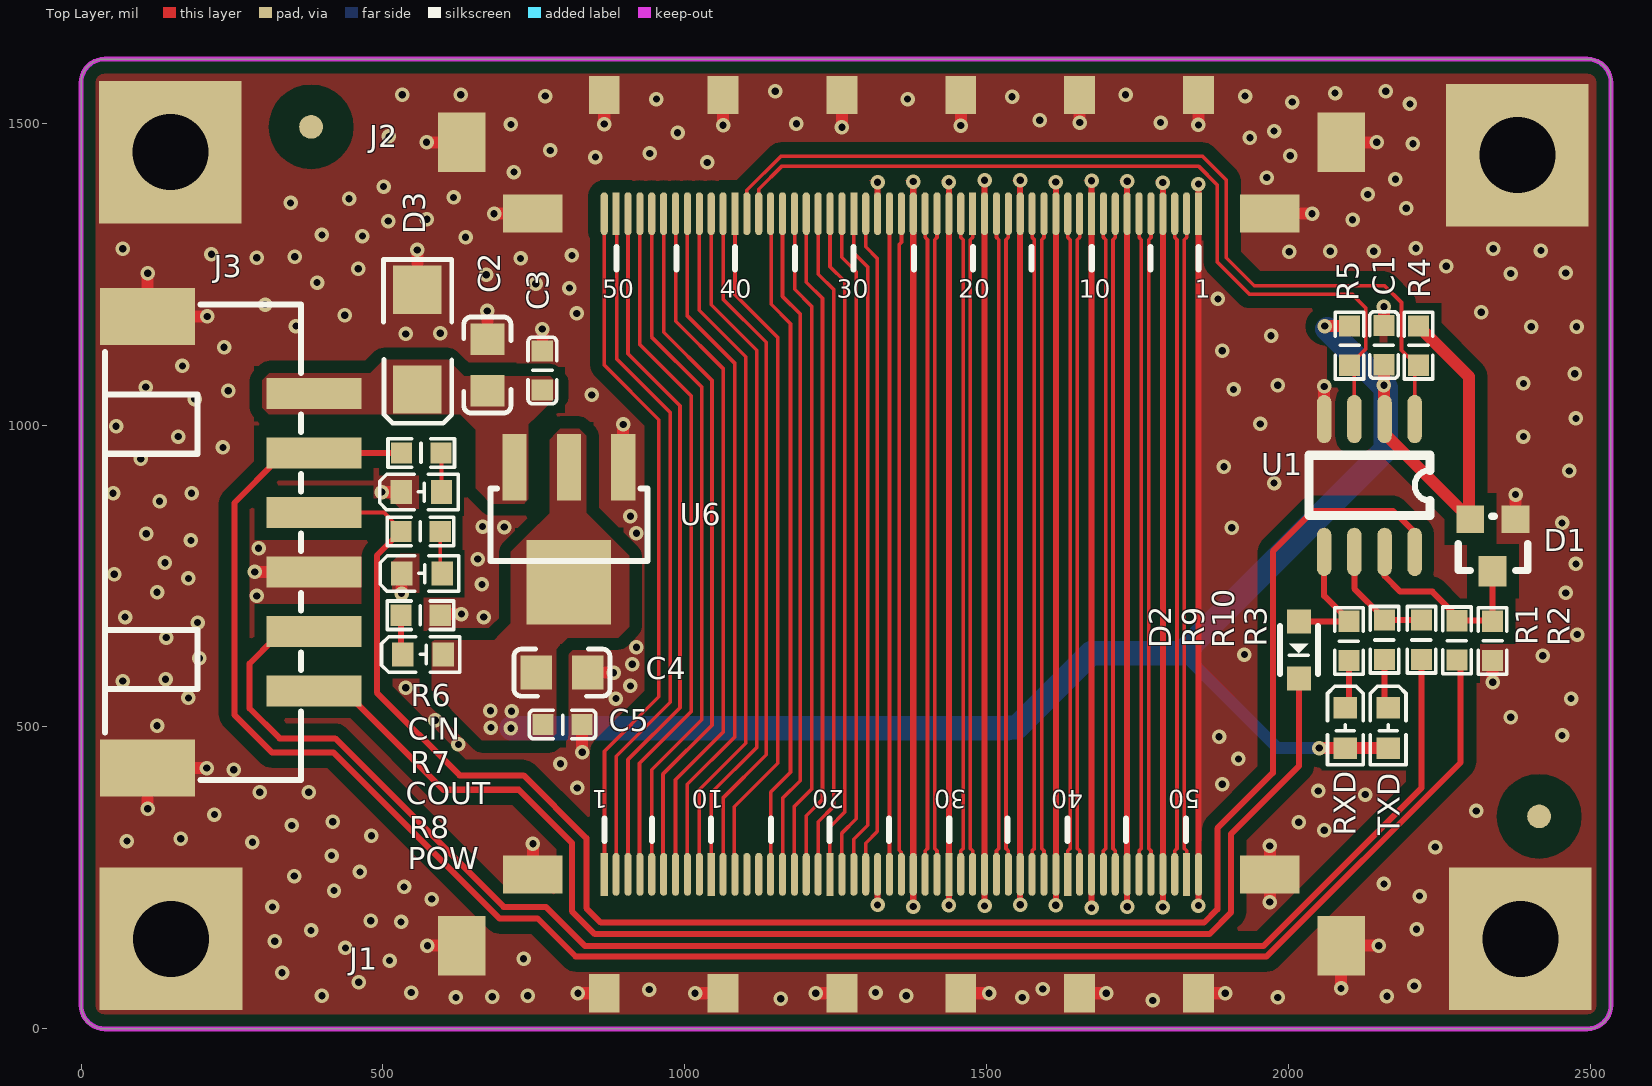
[diagram p0: Top Layer view]
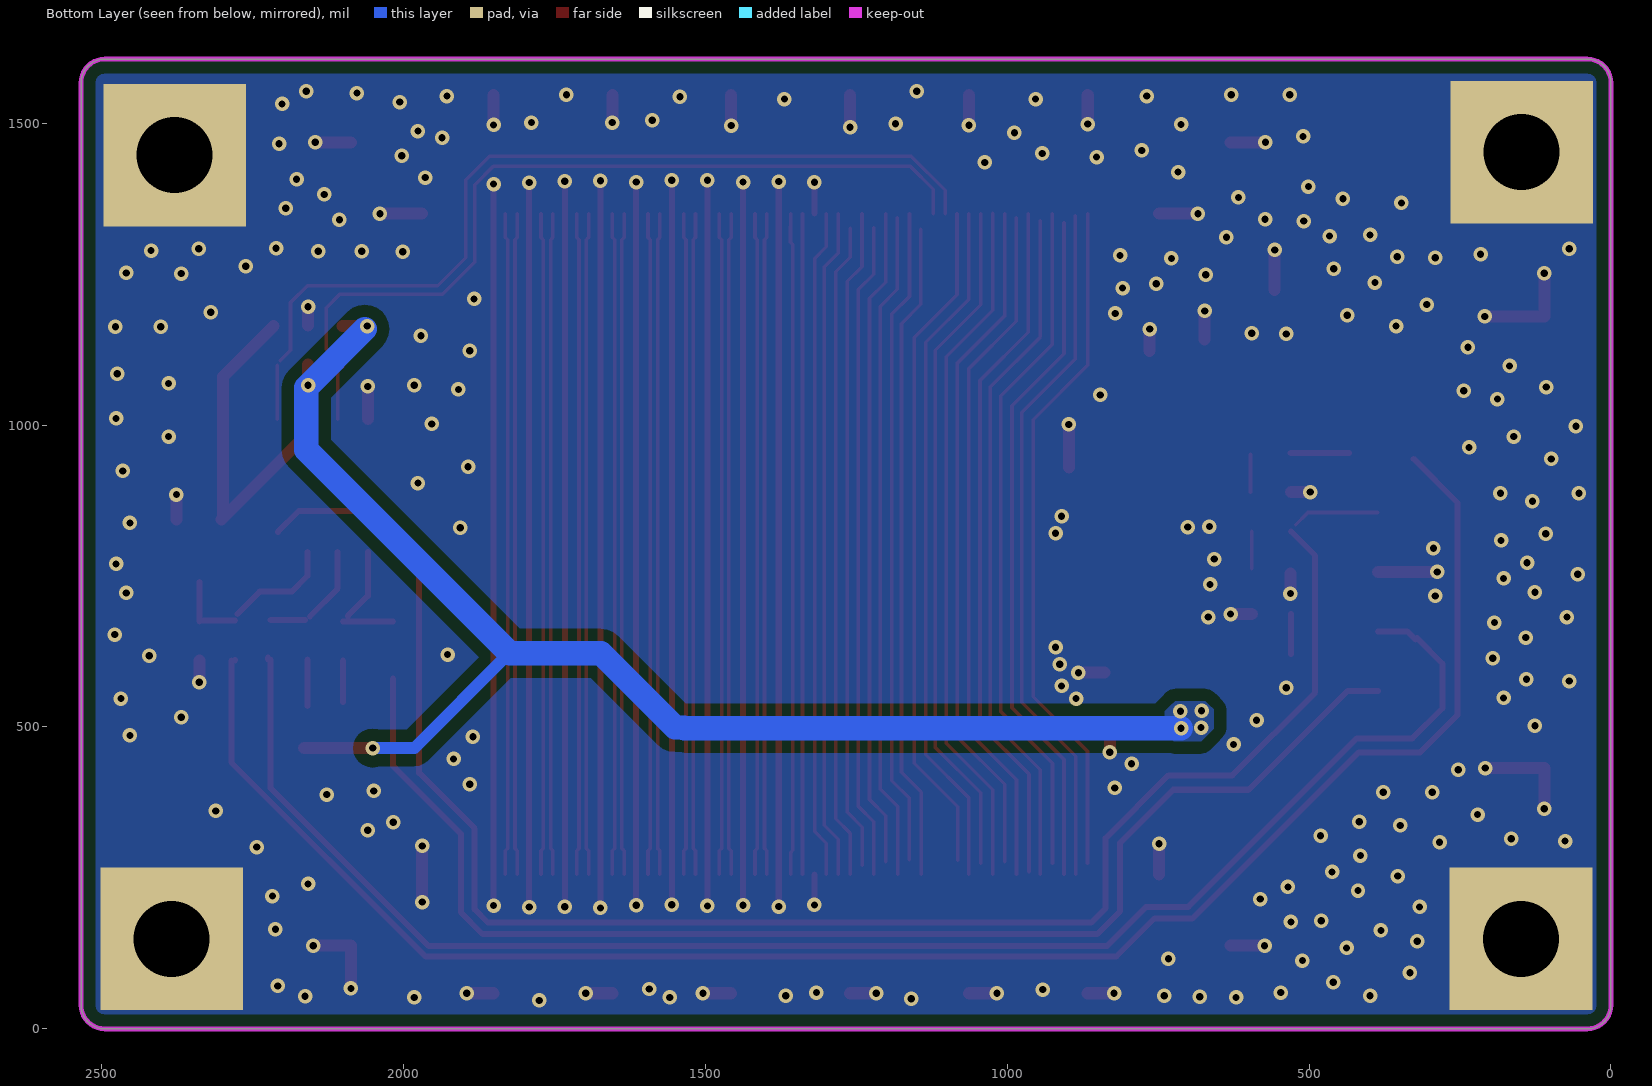
[diagram p1: Bottom Layer view, seen from below]
# Altium PCB MISC80583.PcbDoc
Units mil, origin at the board's own origin, x right, y up, seen from the top; angles counter-clockwise.
Board outline 2534.02 x 1606.3 mil, 2 copper layers (Top Layer, Bottom Layer), stack 12.8 mil thick; 28 components, 56 nets, 195 pads, 259 vias.

## Layer stack, top to bottom
Top Layer: signal copper 1.4
Dielectric: core 10, FR-4, Dk 4.2
Bottom Layer: signal copper 1.4

## Board outline
0,39.37 0,1566.93 cw(c39.37,1566.93) 39.37,1606.3 2494.65,1606.3 cw(c2494.65,1566.93) 2534.02,1566.93 2534,1566.93 2534,39.37 2534.02,39.37 cw(c2494.65,39.37) 2494.65,0 39.37,0 cw(c39.37,39.37)

## Design rules (kind name [scope] priority, off if disabled: settings)
Clearance Clearance_1 [haspad('free-mark')] p1: gap=50
Clearance Clearance_inpoly [inpolygon] p2: gap=20
Clearance [All] p3: gap=6
ComponentClearance [All] p1 off: gap=10 collisioncheckmode=3 verticalgap=10 showdistances=FALSE
DiffPairsRouting [All] p1: maxlimit=40 minlimit=6 mostfreqgap=6 maxuncoupledlength=500
Height [All] p1 off: minheight=0 maxheight=1000 prefheight=500
HoleSize [All] p1 off: absolutevalues=TRUE maxlimit=100 minlimit=1 maxpercent=80.000 minpercent=20.000
MinimumSolderMaskSliver [All] p1 off: minsoldermaskwidth=10
PasteMaskExpansion [All] p1 off: expansion=0
PolygonConnect PolygonConnect_FULL [InPadClass('FULL') Or ISVIA] p1: connectstyle=Direct reliefconductorwidth=10 reliefentries=4 polygonreliefangle="90 Angle"
PolygonConnect [All] p2: connectstyle=Direct reliefconductorwidth=10 reliefentries=4 polygonreliefangle="90 Angle"
RoutingVias [All] p1: holewidth=12 width=24 viastyle="Through Hole" minholewidth=12 minwidth=24 maxholewidth=12 maxwidth=24
SilkToSilkClearance [All] p1 off: silktosilkclearance=10
SilkscreenOverComponentPads SilkToSolderMaskClearance [IsPad] p1 off: minsilkscreentomaskgap=10
SolderMaskExpansion [All] p1 off: expansion=4
Width [All] p1: maxlimit=100 minlimit=6 preferedwidth=6 minimp=50.000000 maximp=50.000000 favimp=50.000000
20 further rules are at their usual default settings.

## Classes and differential pairs
differential pair D7: +D7_P -D7_N
differential pair D6: +D6_P -D6_N
differential pair D5: +D5_P -D5_N
differential pair D4: +D4_P -D4_N
differential pair D3: +D3_P -D3_N
differential pair D2: +D2_P -D2_N
differential pair D1: +D1_P -D1_N
differential pair D0: +D0_P -D0_N

## Components (designator, comment, footprint, x,y, rotation, side; value= is the part's Value field where it differs from the comment)
C1 "0.1uf 50V" 0603C 2158,1165 r270 top
C2 "10uF 16V" 0805C 673,1057 r90 top
C3 "0.1uf 50V" 0603C 764,1058 r90 top
C4 "10uF 16V" 0805C 754,590 r0 top
C5 "0.1uf 50V" 0603C 765,504 r0 top
CIN "LED-RED" LED0603 597,889 r270 top
COUT "LED-RED" LED0603 598,754 r270 top
D1 "BAV99" SOT-23 2376,844 r180 top
D2 "1N5819" SOD-323 2017,627 r270 top
D3 "SMAJ5.0A" 1N5822 557,1224 r270 top
J1 "FPC" FPC-0.5-51P 630,136 r0 top locked
J2 "FPC" FPC-0.5-51P 2087.41,1470 r180 top locked
J3 "CON8" CON6-Lay 386,1052 r270 top
POW "LED-RED" LED0603 600,620 r270 top
R1 "1K" 0603R 2279,676 r270 top
R2 "4.7K" 0603R 2338,610 r90 top
R3 "100R" 0603R 2220,677 r270 top
R4 "4.7K" 0603R 2215,1099 r90 top
R5 "4.7K" 0603R 2101,1099 r90 top
R6 "4.7K" 0603R 596,954 r180 top
R7 "4.7K" 0603R 595,824 r180 top
R8 "4.7K" 0603R 595,685 r180 top
R9 "4.7K" 0603R 2100,675 r270 top
R10 "4.7K" 0603R 2159,677 r270 top
RXD "LED-RED" LED0603 2094,465 r180 top
TXD "LED-RED" LED0603 2165,465 r180 top
U1 "STC8G1K08" so-8 2209,1010 r270 top
U6 "1117-3.3" SOT-223 898,930 r180 top

## Footprints (in the part's own frame and the unit in brackets; to place one, negate y for a bottom-side part, rotate by r counter-clockwise, add the part's x,y. Pads: shape width x height; smd on the part's side, far side on the other; paste and mask are expansions set on the pad)
1N5822 [mil]
  rect 80x80 smd: 1(0,0) 2(165,0)
  silkscreen extent -50,-56 221,57
0603C [mil]
  rect 35x35 smd: 1(0,0) 2(65,0)
  silkscreen extent -23,-24 88,24
0603R [mil]
  rect 35x35 smd: 1(0,0) 2(65,0)
  silkscreen extent -23,-24 88,24
0805C [mil]
  rect 52x56 smd: 1(0,0) 2(85,0)
  silkscreen extent -37,-39 122,39
CON6-Lay [mm]
  rect 1.3x4 smd: 1(0,0) 2(2.5,0) 3(5,0) 4(7.5,0) 5(10,0) 6(12.5,0)
  rect 2.4x4 smd: 7(15.75,-7) 8(-3.25,-7)
  silkscreen extent -3.75,-8.8 16.25,-0.55
FPC-0.5-51P [mm]
  rect 0.3x1.8 smd: 1(6.009,3.044) 10(10.509,3.044) 20(15.509,3.044) 30(20.509,3.044) 40(25.509,3.044) 50(30.509,3.044)
  oval 0.3x1.8 smd: 2(6.509,3.044) 3(7.009,3.044) 4(7.509,3.044) 5(8.009,3.044) 6(8.509,3.044) 7(9.009,3.044) 8(9.509,3.044) 9(10.009,3.044) 11(11.009,3.044) 12(11.509,3.044) 13(12.009,3.044) 14(12.509,3.044) 15(13.009,3.044) 16(13.509,3.044) 17(14.009,3.044) 18(14.509,3.044) 19(15.009,3.044) 21(16.009,3.044) 22(16.509,3.044) 23(17.009,3.044) 24(17.509,3.044) 25(18.009,3.044) 26(18.509,3.044) 27(19.009,3.044) 28(19.509,3.044) 29(20.009,3.044) 31(21.009,3.044) 32(21.509,3.044) 33(22.009,3.044) 34(22.509,3.044) 35(23.009,3.044) 36(23.509,3.044) 37(24.009,3.044) 38(24.509,3.044) 39(25.009,3.044) 41(26.009,3.044) 42(26.509,3.044) 43(27.009,3.044) 44(27.509,3.044) 45(28.009,3.044) 46(28.509,3.044) 47(29.009,3.044) 48(29.509,3.044) 49(30.009,3.044) 51(31.009,3.044)
  rect 2x2.5 smd: 52(0.009,0.044) 52(37.009,0.044)
  rect 2.5x1.6 smd: 52(3.009,3.044) 52(34.009,3.044)
  rect 1.3x1.6 smd: 52(6.009,-1.956) 52(11.009,-1.956) 52(16.009,-1.956) 52(21.009,-1.956) 52(26.009,-1.956) 52(31.009,-1.956)
  silkscreen extent 6.01,4.45 30.49,5.39
LED0603 [mm]
  rect 1x0.9 smd: 1(0,0) 2(0,-1.7)
  silkscreen extent -0.75,-2.6 0.75,0.7
so-8 [mil]
  oval 80x24 smd: 1(0,0) 2(0,-50) 3(0,-100) 4(0,-150) 5(220,-150) 6(220,-100) 7(220,-50) 8(220,0)
  silkscreen extent 60,-175 160,25
SOD-323 [mm]
  rect 1x1 smd: 1(-1.211,0.003) 2(1.189,0.003)
  silkscreen extent -1.01,-0.8 0.99,0.8
SOT-23 [mil]
  rect 46x46 smd: 1(0,0) 2(75,0)
  rect 46x50 smd: 3(38,86)
  silkscreen extent -20,-5 95,85
SOT-223 [mil]
  rect 40x110 smd: 1(0,0) 2(90,0) 3(180,0)
  rect 140x140 smd: 2(90,190)
  silkscreen extent -40,35 220,155

## Part data
C1 C3 C5: library part CAP, "Capacitor"
C2 C4: library part CAPACITOR, "Capacitor"
CIN COUT POW RXD TXD: library part LED2, "Typical RED, GREEN, YELLOW, AMBER GaAs LED"
D3: library part 1N5819
J1 J2: library part FPC-0.5-51P
J3: "Connector"
R1 R2 R3 R4 R5 R6 R7 R8 R9 R10: library part RES2
U6: library part AS1117

## Free pads (board coordinates)
  rect 236.22x236.22 hole 125.98: 0(148,1452) 0(149,149) 0(2379,1447) 0(2384,149)
  round 39.37 smd mask+39.37: MARK(381,1494) MARK(2415,352)

## Via types
v1: diameter 24, hole 12, Top Layer to Bottom Layer, 259 vias

## Nets (pads, with @x,y where several pads share a name; then routed paths per layer and width w, separated by ;. In a path a pad name is that pad's centre, name@x,y a point inside that pad or via, vN(x,y) a via of type N, cw(c..) or ccw(c..) an arc to the next point about the centre after c; other vN are vias at no path point)
CTRL_IN: J3.2 R1.2 R6.2 | length 3050.8
  Top Layer w10: J3.2@327,944 254,871 254,520 316,458 418,458 693,183 756,183 819,120 1963.8,120 2285,441.2 R1.2@2285,610 ; J3.2@434,954 R6.2 ; R1.2@2279,610 R1.2
CTRL_OUT: J3.3 R7.2 U1.8 | length 2962.2
  Top Layer w6: J3.3 501.85,855.15 R7.2@522,835
  Top Layer w10: R7.2 490,784 490,557 627,420 733,420 837,316 837,200 861,176 1860,176 1882,198 1882,332 1974,424 1974,791 2041,858 2173,858 U1.8@2208,823
D0_N: J1.29 J2.23 | length 1097.5
  Top Layer w6: J1.29 1417.76,294.84 1413.92,298.68 1413.92,1307 1417.76,1310.84 J2.23
D0_P: J1.28 J2.24 | length 1097.5
  Top Layer w6: J1.28 1398.07,294.84 1401.92,298.68 1401.92,1307 1398.07,1310.84 J2.24
D1_N: J1.32 J2.20 | length 1097.5
  Top Layer w6: J1.32 1476.81,294.84 1472.97,298.68 1472.97,1307 1476.81,1310.84 J2.20
D1_P: J1.31 J2.21 | length 1097.5
  Top Layer w6: J1.31 1457.13,294.84 1460.97,298.68 1460.97,1307 1457.13,1310.84 J2.21
D2_N: J1.35 J2.17 | length 1097.5
  Top Layer w6: J1.35 1535.87,294.84 1532.03,298.68 1532.03,1307 1535.87,1310.84 J2.17
D2_P: J1.34 J2.18 | length 1097.5
  Top Layer w6: J1.34 1516.18,294.84 1520.03,298.68 1520.03,1307 1516.18,1310.84 J2.18
D3_N: J1.38 J2.14 | length 1097.5
  Top Layer w6: J1.38 1594.92,294.84 1591.08,298.68 1591.08,1307 1594.92,1310.84 J2.14
D3_P: J1.37 J2.15 | length 1097.5
  Top Layer w6: J1.37 1575.24,294.84 1579.08,298.68 1579.08,1307 1575.24,1310.84 J2.15
D4_N: J1.41 J2.11 | length 1097.5
  Top Layer w6: J1.41 1653.98,294.84 1650.14,298.68 1650.14,1307 1653.98,1310.84 J2.11
D4_P: J1.40 J2.12 | length 1097.5
  Top Layer w6: J1.40 1634.29,294.84 1638.14,298.68 1638.14,1307 1634.29,1310.84 J2.12
D5_N: J1.44 J2.8 | length 1097.5
  Top Layer w6: J1.44 1713.03,294.84 1709.19,298.68 1709.19,1307 1713.03,1310.84 J2.8
D5_P: J1.43 J2.9 | length 1097.5
  Top Layer w6: J1.43 1693.35,294.84 1697.19,298.68 1697.19,1307 1693.35,1310.84 J2.9
D6_N: J1.47 J2.5 | length 1097.5
  Top Layer w6: J1.47 1772.09,294.84 1768.25,298.68 1768.25,1307 1772.09,1310.84 J2.5
D6_P: J1.46 J2.6 | length 1097.5
  Top Layer w6: J1.46 1752.4,294.84 1756.25,298.68 1756.25,1307 1752.4,1310.84 J2.6
D7_N: J1.50 J2.2 | length 1097.5
  Top Layer w6: J1.50 1831.14,294.84 1827.3,298.68 1827.3,1307 1831.14,1310.84 J2.2
D7_P: J1.49 J2.3 | length 1097.5
  Top Layer w6: J1.49 1811.46,294.84 1815.3,298.68 1815.3,1307 1811.46,1310.84 J2.3
GND: C1.1 C2.2 C3.2 C4.2 C5.2 CIN.2 COUT.2 D1.1 D3.1 J1.24 J1.27 J1.30 J1.33 J1.36 J1.39 J1.42 J1.45 J1.48 J1.51 J1.52 J2.1 J2.4 J2.7 J2.10 J2.13 J2.16 J2.19 J2.22 J2.25 J2.28 J2.52 J3.4 J3.7 J3.8 pad.0 R2.1 R8.1 U1.4 U6.1 | length 13059.2
  Top Layer w10: v1(1319.33,205.33) J1.24 ; J2.28 v1(1319.33,1402.33) ; v1(1378.39,202.61) J1.27 J2.25 v1(1378.39,1403.39) ; v1(1437.44,204.56) J1.30 J2.22 v1(1437.44,1402.44) ; v1(1496.5,203.5) J1.33 J2.19 v1(1496.5,1405.5) ; v1(1555.55,205.55) J1.36 J2.16 v1(1555.55,1405.55) ; v1(1614.61,204.61) J1.39 J2.13 v1(1614.61,1402.61) ; v1(1673.66,200.34) J1.42 J2.10 v1(1673.66,1404.66) ; v1(1732.72,202.28) J1.45 J2.7 v1(1732.72,1403.72) ; v1(1791.77,201.77) J1.48 J2.4 v1(1791.77,1401.77) ; v1(1850.83,204.17) J1.51 J2.1 v1(1850.83,1399.17)
  Top Layer w20: v1(110.41,364.41) J3.7 v1(208.08,431.92) ; v1(110.41,1251.59) J3.8 v1(208.95,1179.95) ; v1(287.72,756.72) J3.4 ; v1(498,889) CIN.2 ; v1(531,721) 531.07,721.07 COUT.2 ; D3.1 v1(557,1290) ; v1(572.27,1468.27) J2.52@630.36,1468.27 ; v1(573.73,137.73) J1.52@630.36,137.73 ; R8.1@595,687 v1(630,687) ; C2.2 v1(673,1189) ; v1(684.16,1350.16) J2.52@748.47,1350.16 ; J1.52@748.47,255.84 v1(748.47,306.47) ; C3.2 v1(764,1159) ; v1(822.99,58.99) J1.52@866.58,58.99 ; v1(830,458) C5.2 ; C4.2 v1(882,590) ; v1(866.58,1498.58) J2.52@866.58,1547.01 ; U6.1 v1(898,1001) ; v1(1017.01,58.99) J1.52@1063.43,58.99 ; v1(1063.43,1496.57) J2.52@1063.43,1547.01 ; v1(1216.99,58.99) J1.52@1260.28,58.99 ; v1(1260.28,1493.28) J2.52@1260.28,1547.01 ; J1.52@1457.13,58.99 v1(1503.99,58.99) ; v1(1457.13,1496.13) J2.52@1457.13,1547.01 ; J1.52@1653.98,58.99 v1(1698.01,58.99) ; v1(1653.98,1501.02) J2.52@1653.98,1547.01 ; J1.52@1850.83,58.99 v1(1894.99,58.99) ; v1(1850.83,1497.17) J2.52@1850.83,1547.01 ; v1(1968.94,210.06) 1968.94,255.84 v1(1968.94,302.94) ; J2.52@1968.94,1350.16 v1(2038.84,1350.16) ; U1.4 v1(2059,1064) ; v1(2087.05,66.95) 2087.05,137.73 v1(2149.27,137.73) ; J2.52@2087.05,1468.27 v1(2146.27,1468.27) ; C1.1 v1(2158,1196) ; v1(2338,574) R2.1 ; D1.1 v1(2376,885)
  other v1: 1775,47 1159,50 621,52 1559,52 1982,52 681,53 2163,54 399,55 740,55 1367,55 547,60 1316,60 941,65 1593,66 2208,71 460,77 333,93 511,113 733,116 438,134 321,145 381,163 2212,165 530,177 480,179 317,202 581,215 2217,220 419,229 535,235 2158,240 353,253 462,260 415,287 2243,301 284,309 76,311 165,315 481,320 2059,329 349,337 2017,342 417,343 221,355 2311,361 2127,388 296,392 377,392 2049,394 822,399 1890,405 253,429 794,439 1917,447 625,471 1885,484 2453,486 126,502 587,511 2368,516 886,547 2468,547 178,548 538,565 910,568 69,576 140,579 913,604 196,614 2421,618 1927,620 920,632 141,648 2478,653 193,673 73,682 667,682 291,717 2459,722 126,723 664,736 178,746 55,753 2476,770 139,772 657,778 294,796 182,809 108,820 920,821 1906,830 701,831 665,832 2453,838 910,849 130,874 53,887 183,887 1976,904 2465,924 1893,931 99,944 235,963 161,981 2389,981 58,998 1953,1002 2476,1011 188,1043 846,1050 244,1057 1909,1059 107,1063 1982,1066 2389,1069 2474,1085 168,1098 1890,1123 237,1129 1971,1148 538,1151 595,1152 2402,1163 2477,1163 356,1164 437,1182 821,1185 2319,1187 305,1199.64 1883,1209 809,1227 753,1234 391,1236 671,1249 2368,1251 2459,1252 459,1259 2261,1263 728,1276 291,1277 354,1279 813,1281 216,1283 2001,1287 2069,1288 2141,1288 2418,1289 69,1292 2339,1292 2211,1293 637,1311 466,1313 399,1315 509,1338 2106,1340 573,1341 2195,1359 347,1368 444,1375 617,1377 2131,1382 501,1395 2177,1407 1964,1410 717,1419 1037,1435 852,1444 2003,1446 942,1450 777,1455 2206,1466 1936,1476 510,1478 988,1484 1976,1487 712,1498 1185,1499 1788,1501 1588,1505 2201,1532 2006,1535 953,1540 1369,1540 1542,1544 769,1545 1928,1545 532,1547 629,1547 1730,1547 2077,1550 1150,1553 2161,1553
NetCIN_1: CIN.1 R6.1 | length 63
  Top Layer w6: CIN.1 R6.1@597,952
NetCOUT_1: COUT.1 R7.1 | length 62
  Top Layer w6: COUT.1@595,762 R7.1
NetD1_3: D1.3 R1.1 R2.2 U1.7 | length 302.1
  Top Layer w10: U1.7 2159,750 2185,724 2238,724 R1.1@2275,687 ; R1.1 R2.2@2334,676 ; R2.2 D1.3@2338,740
NetJ1_1: J1.1 J2.51 | length 1150.9
  Top Layer w6: J2.51 866.58,1099.42 957,1009 957,550 867,460 J1.1@867,274
NetJ1_2: J1.2 J2.50 | length 1165.2
  Top Layer w6: J1.2 886.26,451.26 976,541 976,1021 887,1110 J2.50@887,1347
NetJ1_3: J1.3 J2.49 | length 1150.4
  Top Layer w6: J1.3 905.95,445.95 992,532 992,1032 906,1118 J2.49@906,1335
NetJ1_4: J1.4 J2.48 | length 1147.1
  Top Layer w6: J1.4@925,274 925,440 1011,526 1011,1048 925.63,1133.37 J2.48
NetJ1_5: J1.5 J2.47 | length 1150.8
  Top Layer w6: J2.47@945,1338 945,1146 1028,1063 1028,512 945.32,429.32 J1.5
NetJ1_6: J1.6 J2.46 | length 1156.8
  Top Layer w6: J1.6@964,260 964,422 1045,503 1045,1074 965,1154 J2.46
NetJ1_7: J1.7 J2.45 | length 1152.7
  Top Layer w6: J1.7 984.69,412.69 1064,492 1064,1093 985,1172 J2.45@985,1343
NetJ1_8: J1.8 J2.44 | length 1138.4
  Top Layer w6: J1.8@1004,277 1004,405 1083,484 1083,1102 1004.37,1180.63 J2.44
NetJ1_9: J1.9 J2.43 | length 1158.9
  Top Layer w6: J2.43@1024,1351 1024,1190 1101,1113 1101,473 1024.06,396.06 J1.9
NetJ1_10: J1.10 J2.42 | length 1138.4
  Top Layer w6: J2.42 1043.74,1199.26 1119,1124 1119,466 1044,391 J1.10@1044,274
NetJ1_11: J1.11 J2.41 | length 1153.6
  Top Layer w6: J1.11 1063.43,382.43 1135,454 1135,1137 1063.43,1208.57 J2.41
NetJ1_12: J1.12 J2.40 | length 1130.3
  Top Layer w6: J1.12@1082,279 1082,368 1154,440 1154,1145 1083.11,1215.89 J2.40
NetJ1_15: J1.15 J2.37 | length 1095
  Top Layer w6: J1.15 1142.17,392.17 1175,425 1175,1168 1143,1200 J2.37@1143,1324
NetJ1_16: J1.16 J2.36 | length 1094.2
  Top Layer w6: J2.36 1161.85,1213.15 1191,1184 1191,411 1162,382 J1.16@1162,280
NetJ1_17: J1.17 J2.35 | length 1110.5
  Top Layer w6: J1.17 1181.54,368.54 1210,397 1210,1197 1182,1225 J2.35@1182,1343
NetJ1_18: J1.18 J2.34 | length 1095.4
  Top Layer w6: J1.18@1201,277 1201,353 1228,380 1228,1210 1201.22,1236.78 J2.34
NetJ1_19: J1.19 J2.33 | length 1092.7
  Top Layer w6: J1.19 1220.91,342.91 1247,369 1247,1224 1221,1250 J2.33@1221,1327
NetJ1_20: J1.20 J2.32 | length 1099.6
  Top Layer w6: J1.20@1240,271 1240,334 1265,359 1265,1238 1240.59,1262.41 J2.32
NetJ1_21: J1.21 J2.31 | length 1089.9
  Top Layer w6: J2.31@1260,1326 1260,1278 1284,1254 1284,348 1260.28,324.28 J1.21
NetJ1_22: J1.22 J2.30 | length 1113.4
  Top Layer w6: J1.22 1279.96,313.96 1303,337 1303,1262 1279.96,1285.04 J2.30
NetJ1_23: J1.23 J2.29 | length 1110.3
  Top Layer w6: J1.23 1299.65,307.65 1319,327 1319,1276 1299.65,1295.35 J2.29
NetJ1_25: J1.25 J2.27 | length 1094.3
  Top Layer w6: J1.25 J2.27
NetJ1_26: J1.26 J2.26 | length 1097.5
  Top Layer w6: J1.26 1358.7,292 1355,295.7 1355,1299 1359,1303 J2.26@1359,1328 ; J2.26@1358.7,1328 J2.26
NetPOW_2: POW.2 R8.2 | length 66
  Top Layer w10: POW.2@530,621 R8.2@530,687
NetR9_2: R9.2 RXD.2 | length 69
  Top Layer w10: RXD.2@2100,541 R9.2
NetR10_2: R10.2 TXD.2 | length 77
  Top Layer w10: TXD.2@2159,535 R10.2
RXD: D2.1 R9.1 U1.5 | length 202.9
  Top Layer w10: D2.1 R9.1@2100.33,674.67 ; U1.5 2059,717 R9.1@2092,684
RXDI: D2.2 J3.6 | length 2200.6
  Top Layer w10: J3.6 436.13,559.87 600,396 725,396 813,308 813,195 851,157 1869,157 1905,193 1905,323 2017.1,435.1 D2.2
SCL: J2.38 R5.1 U1.3 | length 1432.1
  Top Layer w6: J2.38 1122.48,1390.48 1161,1429 1850.7,1429 1882,1397.7 1882,1270 1935,1217 2105,1217 2128,1194 2128,1126 R5.1 ; R5.1@2101,1097 R5.1@2107,1097 ; U1.3 R5.1@2109,1096
SDA: J2.39 R4.1 U1.1 | length 1514
  Top Layer w6: J2.39 1102.8,1388.8 1159,1445 1858,1445 1897,1406 1897,1277 1943,1231 2159,1231 2187,1203 2187,1124 R4.1@2204,1107 ; U1.1 R4.1@2209,1099
TXD: R3.1 R10.1 U1.6 | length 183.1
  Top Layer w10: U1.6 2109,729 R10.1@2155,683 ; R10.1@2163,677 R3.1
TXDI: J3.5 R3.2 | length 2630.4
  Top Layer w10: J3.5@321,647 279,605 279,531 329,481 421,481 700,202 770,202 835,137 1958.17,137 2220,398.83 R3.2 ; J3.5@323.5,644.5 337.3,658.3 J3.5 ; R3.2@2224,612 R3.2@2224,615
VCC_3.3V: C1.2 C4.1 C5.1 D1.2 POW.1 R4.2 R5.2 RXD.1 TXD.1 U1.2 U6.2 | length 2991.5
  Top Layer w20: v1(2051,465) RXD.1 ; v1(2060,1164) R5.2 ; RXD.1@2087,465 RXD.1 ; U1.2@2158,1035 v1(2158,1066) C1.2 ; U1.2@2160,1028 2160,985 D1.2 ; TXD.1 RXD.1 ; R4.2 2299,1080 D1.2@2299,851
  Bottom Layer w20: 1827,620 1982,465 v1(2051,465) ; v1(2060,1164) v1@2064.5,1159.5
  Bottom Layer w40: v1(712,498) 1535,498 ; 1535,499 1550,499 1673,622 1824,622 2161,959 2161,1062 v1@2064,1159
  other v1: 679,499 713,526 678,527
VCC_5V: C2.1 C3.1 D3.2 J3.1 U6.3
pads on no net: J1.13 J1.14

## Polygon pours and split planes (outlines as drawn)
GND on Top Layer "BottomLayer-No Net" (solid, remove dead copper): -86.55,1599.79 -55.55,1568.79 -55.55,-59.21 2547.45,-59.21 2606.45,-0.21 2638.45,31.79 2638.45,1100.79 2638.45,1593.79 2553.45,1678.79 2525.45,1706.79 2242.45,1706.79 -21.55,1706.79 -77.55,1650.79 -83.55,1644.79 -83.55,1618.79
VCC_3.3V on Top Layer "BottomLayer-No Net" (solid, remove dead copper): 776,957 776,854 741,819 712,790 712,750 712,672 694,654 684,644 616,644 585,644 582,641 581,640 581,637 581,561 614,528 664,478 735,478 776,478 781,483 787,489 787,495 787,629 796,638 806,648 834,648 890,648 899,657 908,666 908,692 908,784 865,827 837,855 837,911 837,982 827,992 825,994 814,994 794,994 788,988 776,976 776,957
VCC_5V on Top Layer "BottomLayer-No Net" (solid, remove dead copper): 300,1064 300,1040 300,1029 307,1022 311,1018 327,1018 628,1018 653,993 654,992 654,946 654,895 661,888 679,870 683,870 734,870 737,873 741,877 741,887 741,1001 754,1014 787,1047 787,1056 787,1071 781,1077 777,1081 763,1081 635,1081 619,1097 608,1108 564,1108 501,1108 490,1097 479,1086 360,1086 312,1086 307,1081 300,1074 300,1066
GND on Bottom Layer "BottomLayer-No Net" (solid, remove dead copper): -64,1609 -64,-19 -14,-69 7,-90 141,-90 2601,-90 2647,-44 2697,6 2697,1508 2697,1643 2622,1718 2547,1793 2379,1793 125,1793 -55,1613
VCC_3.3V on Bottom Layer "BottomLayer-No Net" (solid, remove dead copper): 658,525 658,497 666,489 679,476 694,476 724,476 729,481 739,491 739,503 739,526 729,536 722,543 714,543 672,543 666,537 658,529 658,525

## Keep-outs
Keep-Out Layer:
  the board outline again, w8